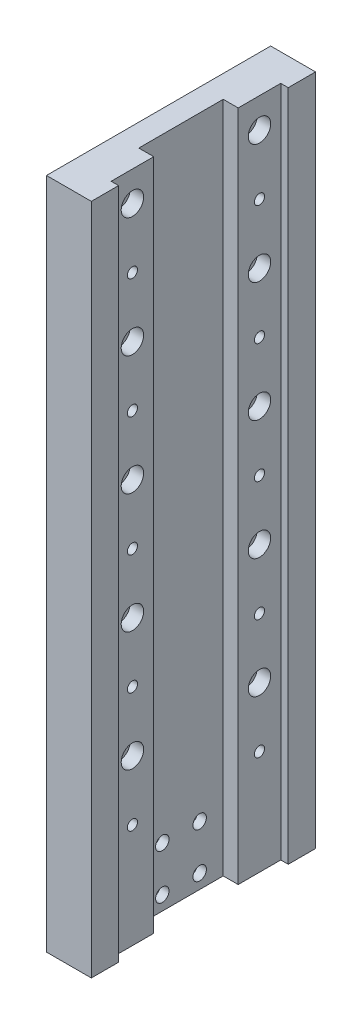
SolidWorks part; units mm, degrees
ref_plane "前视基准面" through (0, 0, 0) normal (0, 0, 1) x (1, 0, 0)
ref_plane "上视基准面" through (0, 0, 0) normal (0, 1, 0) x (1, 0, 0)
ref_plane "右视基准面" through (0, 0, 0) normal (1, 0, 0) x (0, 0, -1)
sketch "草图1" plane through (0, 0, 0) normal (1, 0, 0) x (0, 0, -1)
  line L1 (-75, 225) -> (75, 225)
  line L2 (-75, 225) -> (-75, -225)
  line L3 (-75, -225) -> (75, -225)
  line L4 (75, 225) -> (75, -225)
  line L5 (-75, 225) -> (75, -225) construction
  line L6 (-75, -225) -> (75, 225) construction
  point P0 (0, 0)
  dimension "D1" = 150
  dimension "D2" = 450
extrude "凸台-拉伸1" add sketch "草图1" along normal blind 30
sketch "草图2" plane through (30, 0, 0) normal (1, 0, 0) x (0, 0, -1)
  line L0 (-75, -225) -> (75, -225) construction
  line L1 (-56.75, 225) -> (-28.25, 225)
  line L2 (-56.75, 225) -> (-56.75, -225)
  line L3 (-56.75, -225) -> (-28.25, -225)
  line L4 (-28.25, 225) -> (-28.25, -225)
  line L5 (-56.75, 225) -> (-28.25, -225) construction
  line L6 (-56.75, -225) -> (-28.25, 225) construction
  line L7 (0, 0) -> (0, -84.7426) construction
  line L8 (28.25, 225) -> (56.75, 225)
  line L9 (28.25, 225) -> (28.25, -225)
  line L10 (28.25, -225) -> (56.75, -225)
  line L11 (56.75, 225) -> (56.75, -225)
  line L12 (28.25, 225) -> (56.75, -225) construction
  line L13 (28.25, -225) -> (56.75, 225) construction
  point P0 (-42.5, 0)
  point P7 (42.5, 0)
  dimension "D1" = 85
  dimension "D2" = 28.5
extrude "切除-拉伸1" cut sketch "草图2" against normal blind 5
hole_wizard "M8 螺纹孔1" positions "草图3" profile "草图4" tap size "M8" standard "GB" end condition through all
sketch "草图3" plane through (30, 0, 0) normal (1, 0, 0) x (0, 0, -1)
  line L0 (-42.5, -225) -> (-42.5, -145.0716) construction
  line L1 (-56.75, -225) -> (-28.25, -225) construction
  line L3 (42.5, -225) -> (42.5, -152.7934) construction
  line L4 (28.25, -225) -> (56.75, -225) construction
  point P0 (-42.5, -155)
  point P2 (42.5, -155)
  dimension "D1" = 70
sketch "草图4" plane through (30, -155, 42.5) normal (0, 1, 0) x (0, 0, -1)
  line L0 (0, 0) -> (0, 30)
  line L1 (0, 30) -> (3.4, 30)
  line L2 (3.4, 30) -> (3.4, 0)
  line L5 (3.4, 0) -> (0, 0)
  line L11 (0, -6.35) -> (0, 107.95) construction
  dimension "通孔螺纹孔钻头直径" = 6.8
  dimension "通孔螺纹孔钻头深度" = 30
cosmetic thread "孔螺蚊线1" parameters "D2"=8
cosmetic thread "孔螺蚊线2" parameters "D2"=8
pattern_linear "阵列(线性)1" count 5 spacing 80 along (0, 1, 0) of "M8 螺纹孔1"
hole_wizard "打孔尺寸(%根据)内六角圆柱头螺钉的类型1" positions "草图5" profile "草图6" counterbore size "M8" standard "GB" end condition through all
sketch "草图5" plane through (25, 0, 0) normal (1, 0, 0) x (0, 0, -1)
  line L1 (-42.5, -155) -> (-42.5, -114.26) construction
  line L3 (42.5, -155) -> (42.5, -114.26) construction
  line L5 (-56.75, -225) -> (-28.25, -225) construction
  point P0 (-42.5, -115)
  point P2 (42.5, -115)
  dimension "D1" = 110
sketch "草图6" plane through (25, -115, 42.5) normal (0, 1, 0) x (0, 0, -1)
  line L0 (0, 0) -> (0, 25)
  line L1 (0, 25) -> (4.5, 25)
  line L3 (4.5, 25) -> (4.5, 9)
  line L4 (4.5, 9) -> (7.5, 9)
  line L5 (7.5, 9) -> (7.5, 0)
  line L7 (7.5, 0) -> (0, 0)
  line L11 (0, -6.35) -> (0, 107.95) construction
  dimension "通孔孔直径" = 9
  dimension "通孔孔深度" = 25
  dimension "柱形沉头孔直径" = 15
  dimension "柱形沉头孔深度" = 9
pattern_linear "阵列(线性)2" count 5 spacing 80 along (0, 1, 0) of "打孔尺寸(%根据)内六角圆柱头螺钉的类型1"
sketch "草图7" plane through (30, 0, 0) normal (1, 0, 0) x (0, 0, -1)
  line L0 (-28.25, -225) -> (-28.25, 225) construction
  line L1 (-28.25, 225) -> (28.25, 225)
  line L2 (-28.25, 225) -> (-28.25, -225)
  line L3 (-28.25, -225) -> (28.25, -225)
  line L4 (28.25, 225) -> (28.25, -225)
  dimension "D1" = 450
extrude "切除-拉伸2" cut sketch "草图7" against normal blind 15
hole_wizard "打孔尺寸(%根据)内六角圆柱头螺钉的类型2" positions "草图8" profile "草图9" counterbore size "M8" standard "GB" end condition through all
sketch "草图8" plane through (0, 0, 0) normal (1, 0, 0) x (0, 0, -1)
  line L1 (0, -225) -> (0, -168.3558) construction
  line L2 (-28.25, -225) -> (28.25, -225) construction
  point P0 (-12.5, -185.5)
  point P2 (12.5, -185.5)
  point P4 (-12.5, -215.5)
  point P6 (12.5, -215.5)
  dimension "D1" = 25
  dimension "D2" = 30
  dimension "D3" = 9.5
sketch "草图9" plane through (0, -185.5, 12.5) normal (0, 1, 0) x (0, 0, 1)
  line L0 (0, 0) -> (0, 30)
  line L1 (0, 30) -> (4.5, 30)
  line L3 (4.5, 30) -> (4.5, 9)
  line L4 (4.5, 9) -> (7.5, 9)
  line L5 (7.5, 9) -> (7.5, 0)
  line L7 (7.5, 0) -> (0, 0)
  line L11 (0, -6.35) -> (0, 107.95) construction
  dimension "通孔孔直径" = 9
  dimension "通孔孔深度" = 30
  dimension "柱形沉头孔直径" = 15
  dimension "柱形沉头孔深度" = 9
